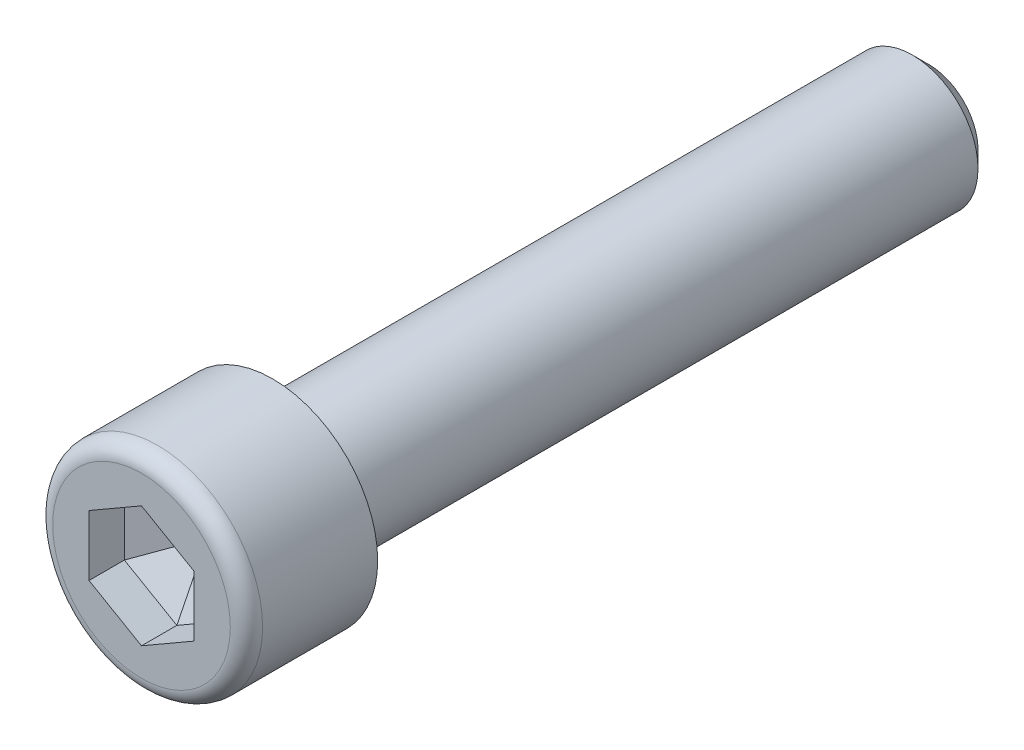
from build123d import *
from OCP.BRepFilletAPI import BRepFilletAPI_MakeChamfer

# Parameters (mm, degrees)
SKETCH1_R           = 8
BOSS_EXTRUDE1_DEPTH = 10
CUT_EXTRUDE1_DEPTH  = 5
SKETCH3_R           = 5
BOSS_EXTRUDE2_DEPTH = 50
CHAMFER1_SIZE       = 1.25
FILLET1_R           = 1.230769231
CHAMFER2_SIZE       = 2.305475504
CHAMFER2_SIZE2      = 3.993200709
FILLET2_R           = 0.1


with BuildPart() as part:
    # Sketch1 → Boss-Extrude1 (new body)
    with BuildSketch(Plane.XY):
        Circle(SKETCH1_R)
    extrude(amount=BOSS_EXTRUDE1_DEPTH)

    # Sketch2 → Cut-Extrude1 (cut)
    with BuildSketch(Plane.XY.offset(10)):
        Polygon((4, 2.309401077), (0, 4.618802154), (-4, 2.309401077), (-4, -2.309401077), (0, -4.618802154), (4, -2.309401077), align=None)
    extrude(amount=-CUT_EXTRUDE1_DEPTH, mode=Mode.SUBTRACT)

    # Sketch3 → Boss-Extrude2 (add)
    with BuildSketch(Plane(origin=(0, 0, 0), x_dir=(-1, 0, 0), z_dir=(0, 0, -1))):
        with Locations(Location((0, 0, 0), (0, 0, 180))):
            Circle(SKETCH3_R)
    extrude(amount=BOSS_EXTRUDE2_DEPTH)

    # Chamfer1
    chamfer1_edges = [part.edges().sort_by_distance(p)[0] for p in [
        (-5, 0, -50),
    ]]
    chamfer(chamfer1_edges, length=CHAMFER1_SIZE)

    # Fillet1
    fillet1_edges = [part.edges().sort_by_distance(p)[0] for p in [
        (-8, 0, 10),
    ]]
    fillet(fillet1_edges, radius=FILLET1_R)

    # Chamfer2: one chamfer whose edges measure the first distance from different faces: ONE call of the kernel's chamfer builder (chamfer() names one face for all edges)
    chamfer2_edges_1 = [part.edges().sort_by_distance(p)[0] for p in [
        (-2, 3.464101615, 5),
    ]]
    chamfer2_side_1 = [part.faces().sort_by_distance(p)[0] for p in [
        (-2, 3.464101615, 7.5),
    ]]
    chamfer2_edges_2 = [part.edges().sort_by_distance(p)[0] for p in [
        (2, 3.464101615, 5),
    ]]
    chamfer2_side_2 = [part.faces().sort_by_distance(p)[0] for p in [
        (2, 3.464101615, 7.5),
    ]]
    chamfer2_edges_3 = [part.edges().sort_by_distance(p)[0] for p in [
        (4, 0, 5),
    ]]
    chamfer2_side_3 = [part.faces().sort_by_distance(p)[0] for p in [
        (4, 0, 7.5),
    ]]
    chamfer2_edges_4 = [part.edges().sort_by_distance(p)[0] for p in [
        (2, -3.464101615, 5),
    ]]
    chamfer2_side_4 = [part.faces().sort_by_distance(p)[0] for p in [
        (2, -3.464101615, 7.5),
    ]]
    chamfer2_edges_5 = [part.edges().sort_by_distance(p)[0] for p in [
        (-2, -3.464101615, 5),
    ]]
    chamfer2_side_5 = [part.faces().sort_by_distance(p)[0] for p in [
        (-2, -3.464101615, 7.5),
    ]]
    chamfer2_edges_6 = [part.edges().sort_by_distance(p)[0] for p in [
        (-4, 0, 5),
    ]]
    chamfer2_side_6 = [part.faces().sort_by_distance(p)[0] for p in [
        (-4, 0, 7.5),
    ]]
    chamfer2 = BRepFilletAPI_MakeChamfer(part.part.solid().wrapped)
    for e in chamfer2_edges_1:
        chamfer2.Add(CHAMFER2_SIZE, CHAMFER2_SIZE2, e.wrapped, chamfer2_side_1[0].wrapped)  # the first distance lies on this face
    for e in chamfer2_edges_2:
        chamfer2.Add(CHAMFER2_SIZE, CHAMFER2_SIZE2, e.wrapped, chamfer2_side_2[0].wrapped)  # the first distance lies on this face
    for e in chamfer2_edges_3:
        chamfer2.Add(CHAMFER2_SIZE, CHAMFER2_SIZE2, e.wrapped, chamfer2_side_3[0].wrapped)  # the first distance lies on this face
    for e in chamfer2_edges_4:
        chamfer2.Add(CHAMFER2_SIZE, CHAMFER2_SIZE2, e.wrapped, chamfer2_side_4[0].wrapped)  # the first distance lies on this face
    for e in chamfer2_edges_5:
        chamfer2.Add(CHAMFER2_SIZE, CHAMFER2_SIZE2, e.wrapped, chamfer2_side_5[0].wrapped)  # the first distance lies on this face
    for e in chamfer2_edges_6:
        chamfer2.Add(CHAMFER2_SIZE, CHAMFER2_SIZE2, e.wrapped, chamfer2_side_6[0].wrapped)  # the first distance lies on this face
    add(Compound.cast(chamfer2.Shape()), mode=Mode.REPLACE)

    # Fillet2
    fillet2_edges = [part.edges().sort_by_distance(p)[0] for p in [
        (-5, 0, 0),
    ]]
    fillet(fillet2_edges, radius=FILLET2_R)


solid = part.part
